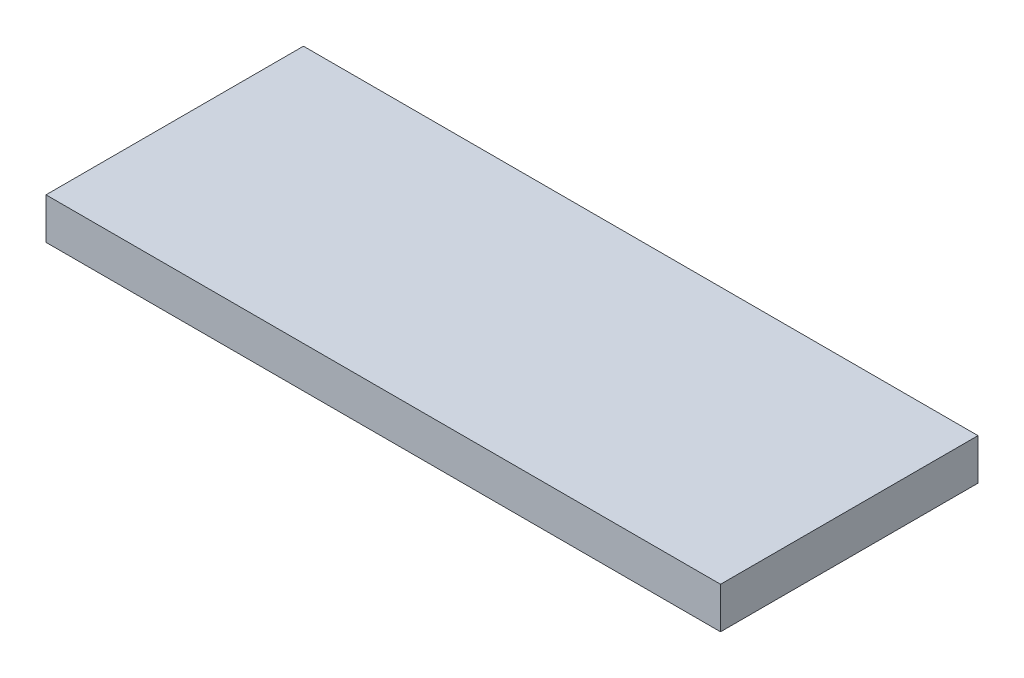
SolidWorks part; units mm, degrees
ref_plane "Front Plane" through (0, 0, 0) normal (0, 0, 1) x (1, 0, 0)
ref_plane "Top Plane" through (0, 0, 0) normal (0, 1, 0) x (1, 0, 0)
ref_plane "Right Plane" through (0, 0, 0) normal (1, 0, 0) x (0, 0, -1)
sketch "Sketch1" plane through (0, 0, 0) normal (0, 0, 1) x (1, 0, 0)
  line L1 (0, 0) -> (131, 0)
  line L2 (0, 0) -> (0, 8)
  line L3 (0, 8) -> (131, 8)
  line L4 (131, 0) -> (131, 8)
  dimension "D1" = 131
  dimension "D2" = 8
extrude "Boss-Extrude1" add sketch "Sketch1" along normal blind 50
sketch "Sketch2" plane through (0, 0, 0) normal (0, 0, -1) x (-1, 0, 0)
  circle A0 centre (-122.3912, 4) radius 2
  circle A1 centre (-85.3912, 4) radius 2
  circle A2 centre (-48.3912, 4) radius 2
  circle A3 centre (-11.3912, 4) radius 2
  dimension "D1" = 4
extrude "Cut-Extrude1" cut sketch "Sketch2" against normal blind 15
